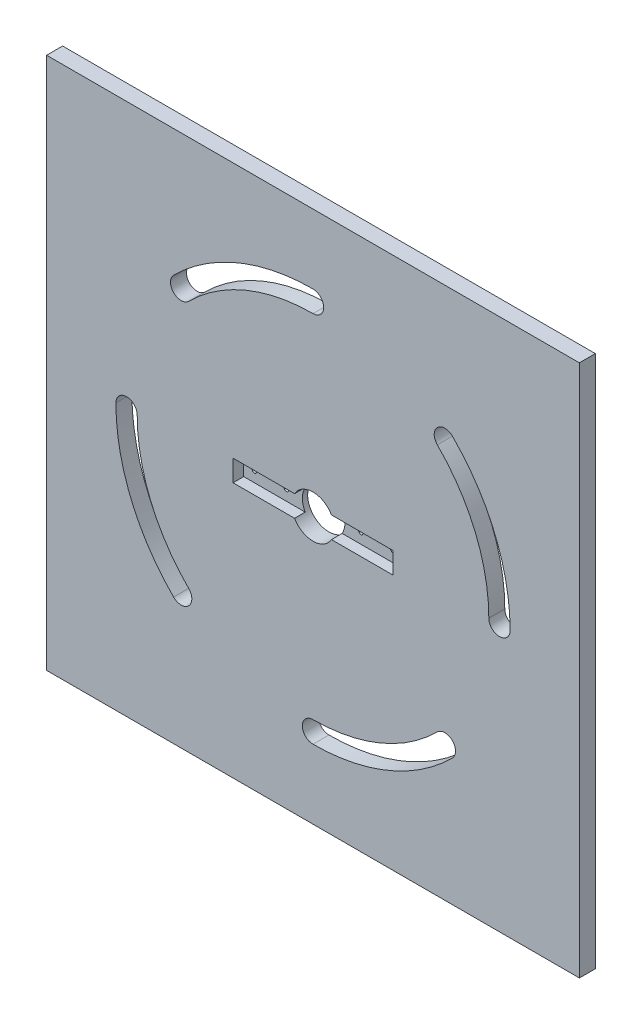
from build123d import *

# Parameters (mm, degrees)
SKETCH1_W           = 1000
SKETCH1_H           = 1000
BOSS_EXTRUDE1_DEPTH = 30
CUT_EXTRUDE1_DEPTH  = 708.742891169
SKETCH3_R           = 40
CUT_EXTRUDE2_DEPTH  = 708.742891169
SKETCH4_W           = 120
SKETCH4_H           = 40
CUT_EXTRUDE3_DEPTH  = 20
M10_TAPPED_HOLE1_D  = 8.5


with BuildPart() as part:
    # Sketch1 → Boss-Extrude1 (new body)
    with BuildSketch(Plane.XY):
        Rectangle(SKETCH1_W, SKETCH1_H)
    extrude(amount=BOSS_EXTRUDE1_DEPTH)

    # Sketch2 → Cut-Extrude1 (cut, through all)
    with BuildSketch(Plane.XY.offset(30)):
        with BuildLine():
            ThreePointArc((0, 370), (-141.592869975, 341.835427029), (-261.629509039, 261.629509039))
            ThreePointArc((-261.629509039, 261.629509039), (-261.629509039, 233.345237792), (-233.345237792, 233.345237792))
            ThreePointArc((-233.345237792, 233.345237792), (-126.28553268, 304.880245729), (0, 330))
            ThreePointArc((0, 330), (20, 350), (0, 370))
        make_face()
        with BuildLine():
            ThreePointArc((370, 0), (341.835427029, 141.592869975), (261.629509039, 261.629509039))
            ThreePointArc((261.629509039, 261.629509039), (233.345237792, 261.629509039), (233.345237792, 233.345237792))
            ThreePointArc((233.345237792, 233.345237792), (304.880245729, 126.28553268), (330, 0))
            ThreePointArc((330, 0), (350, -20), (370, 0))
        make_face()
        with BuildLine():
            ThreePointArc((0, -370), (141.592869975, -341.835427029), (261.629509039, -261.629509039))
            ThreePointArc((261.629509039, -261.629509039), (261.629509039, -233.345237792), (233.345237792, -233.345237792))
            ThreePointArc((233.345237792, -233.345237792), (126.28553268, -304.880245729), (0, -330))
            ThreePointArc((0, -330), (-20, -350), (0, -370))
        make_face()
        with BuildLine():
            ThreePointArc((-370, 0), (-341.835427029, -141.592869975), (-261.629509039, -261.629509039))
            ThreePointArc((-261.629509039, -261.629509039), (-233.345237792, -261.629509039), (-233.345237792, -233.345237792))
            ThreePointArc((-233.345237792, -233.345237792), (-304.880245729, -126.28553268), (-330, 0))
            ThreePointArc((-330, 0), (-350, 20), (-370, 0))
        make_face()
    extrude(amount=-CUT_EXTRUDE1_DEPTH, mode=Mode.SUBTRACT)

    # Sketch3 → Cut-Extrude2 (cut, through all)
    with BuildSketch(Plane.XY.offset(30)):
        Circle(SKETCH3_R)
    extrude(amount=-CUT_EXTRUDE2_DEPTH, mode=Mode.SUBTRACT)

    # Sketch4 → Cut-Extrude3 (cut)
    with BuildSketch(Plane.XY.offset(30)):
        with Locations((-90, 0)):
            Rectangle(SKETCH4_W, SKETCH4_H)
        with Locations((90, 0)):
            Rectangle(SKETCH4_W, SKETCH4_H)
    extrude(amount=-CUT_EXTRUDE3_DEPTH, mode=Mode.SUBTRACT)

    # M10 Tapped Hole1 (through all)
    with Locations(Plane.XY.offset(10)):
        with Locations((-130, 0), (-70, 0), (70, 0), (130, 0)):
            Hole(M10_TAPPED_HOLE1_D / 2)


solid = part.part
